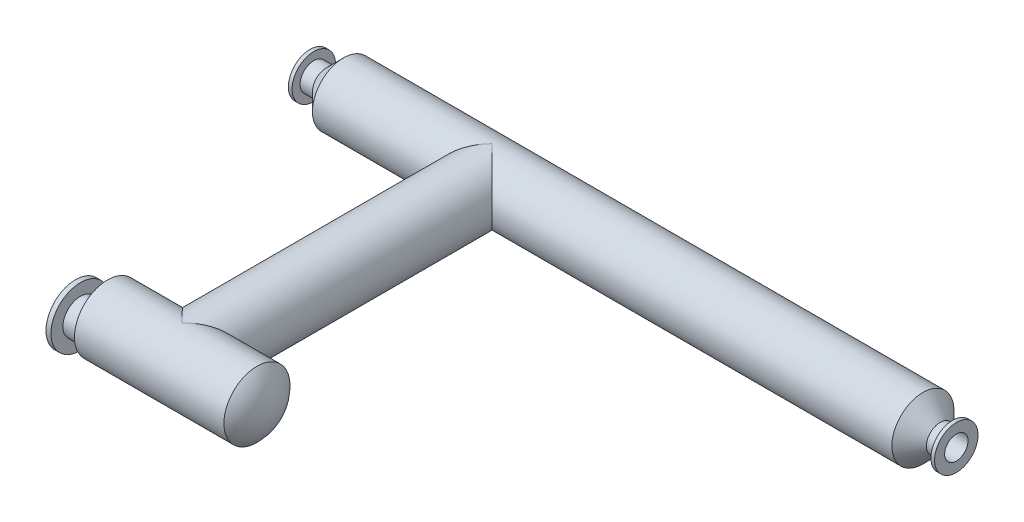
from build123d import *

# Parameters (mm, degrees)
SKETCH2_R           = 150
SKETCH2_R_2         = 140
BOSS_EXTRUDE1_DEPTH = 1500
SKETCH5_R           = 85
SKETCH5_R_2         = 75
BOSS_EXTRUDE2_DEPTH = 100
SKETCH6_R           = 142.5
SKETCH6_R_2         = 60.5
BOSS_EXTRUDE3_DEPTH = 24


with BuildPart() as part:
    # Sketch1 → Revolve1 (revolve)
    with BuildSketch(Plane.XY, mode=Mode.PRIVATE) as revolve1_sk:
        Polygon((0, 56.5), (0, 105), (18, 105), (18, 66.5), (78, 66.5), (161.5, 150), (2962.5, 150), (3046, 66.5), (3106, 66.5), (3106, 105), (3124, 105), (3124, 56.5), (3041.857864376, 56.5), (2958.357864376, 140), (165.642135624, 140), (82.142135624, 56.5), align=None)
    revolve(revolve1_sk.sketch.rotate(Axis((0, 0, 0), (1, 0, 0)), 90), axis=Axis((0, 0, 0), (1, 0, 0)))

    # Sketch2 → Boss-Extrude1 (add)
    with BuildSketch(Plane.XY):
        with Locations((880, 0)):
            Circle(SKETCH2_R)
        with Locations((880, 0)):
            Circle(SKETCH2_R_2, mode=Mode.SUBTRACT)
    extrude(amount=BOSS_EXTRUDE1_DEPTH)

    # Sketch4 → Revolve2 (revolve)
    with BuildSketch(Plane.XY.offset(1500), mode=Mode.PRIVATE) as revolve2_sk:
        with BuildLine():
            Line((1243.197122588, 150), (520.75, 150))
            ThreePointArc((520.75, 150), (503.695994, 70.891478966), (497.200641447, -9.773306511))
            Line((497.200641447, -9.773306511), (507.201689691, -9.773306511))
            ThreePointArc((507.201689691, -9.773306511), (513.061784712, 65.778136969), (528.341718403, 140))
            Line((528.341718403, 140), (1239.100117121, 140))
            ThreePointArc((1239.100117121, 140), (1284.370508191, 71.230087806), (1299.106832019, -9.773306511))
            Line((1299.106832019, -9.773306511), (1309.108967154, -9.773306511))
            ThreePointArc((1309.108967154, -9.773306511), (1292.823288675, 76.990381103), (1243.197122588, 150))
        make_face()
    revolve(revolve2_sk.sketch.rotate(Axis((497.200641447, -9.773306511, 1500), (1, 0, 0)), 90), axis=Axis((497.200641447, -9.773306511, 1500), (1, 0, 0)))



with BuildPart() as body_2:
    # Sketch5 → Boss-Extrude2 (new body)
    with BuildSketch(Plane(origin=(550, 0, 0), x_dir=(0, 0, -1), z_dir=(1, 0, 0))):
        with Locations((-1559.992108681, -8.800220718)):
            Circle(SKETCH5_R)
        with Locations((-1559.992108681, -8.800220718)):
            Circle(SKETCH5_R_2, mode=Mode.SUBTRACT)
    extrude(amount=-BOSS_EXTRUDE2_DEPTH)


with BuildPart() as part_1:
    add(part.part)

    add(body_2.part)  # Boss-Extrude3 merges body 2
    # Sketch6 → Boss-Extrude3 (add)
    with BuildSketch(Plane.ZY.offset(-450)):
        with Locations((1559.992108681, -8.800220718)):
            Circle(SKETCH6_R)
        with Locations((1559.992108681, -8.800220718)):
            Circle(SKETCH6_R_2, mode=Mode.SUBTRACT)
    extrude(amount=BOSS_EXTRUDE3_DEPTH)


solid = part_1.part
